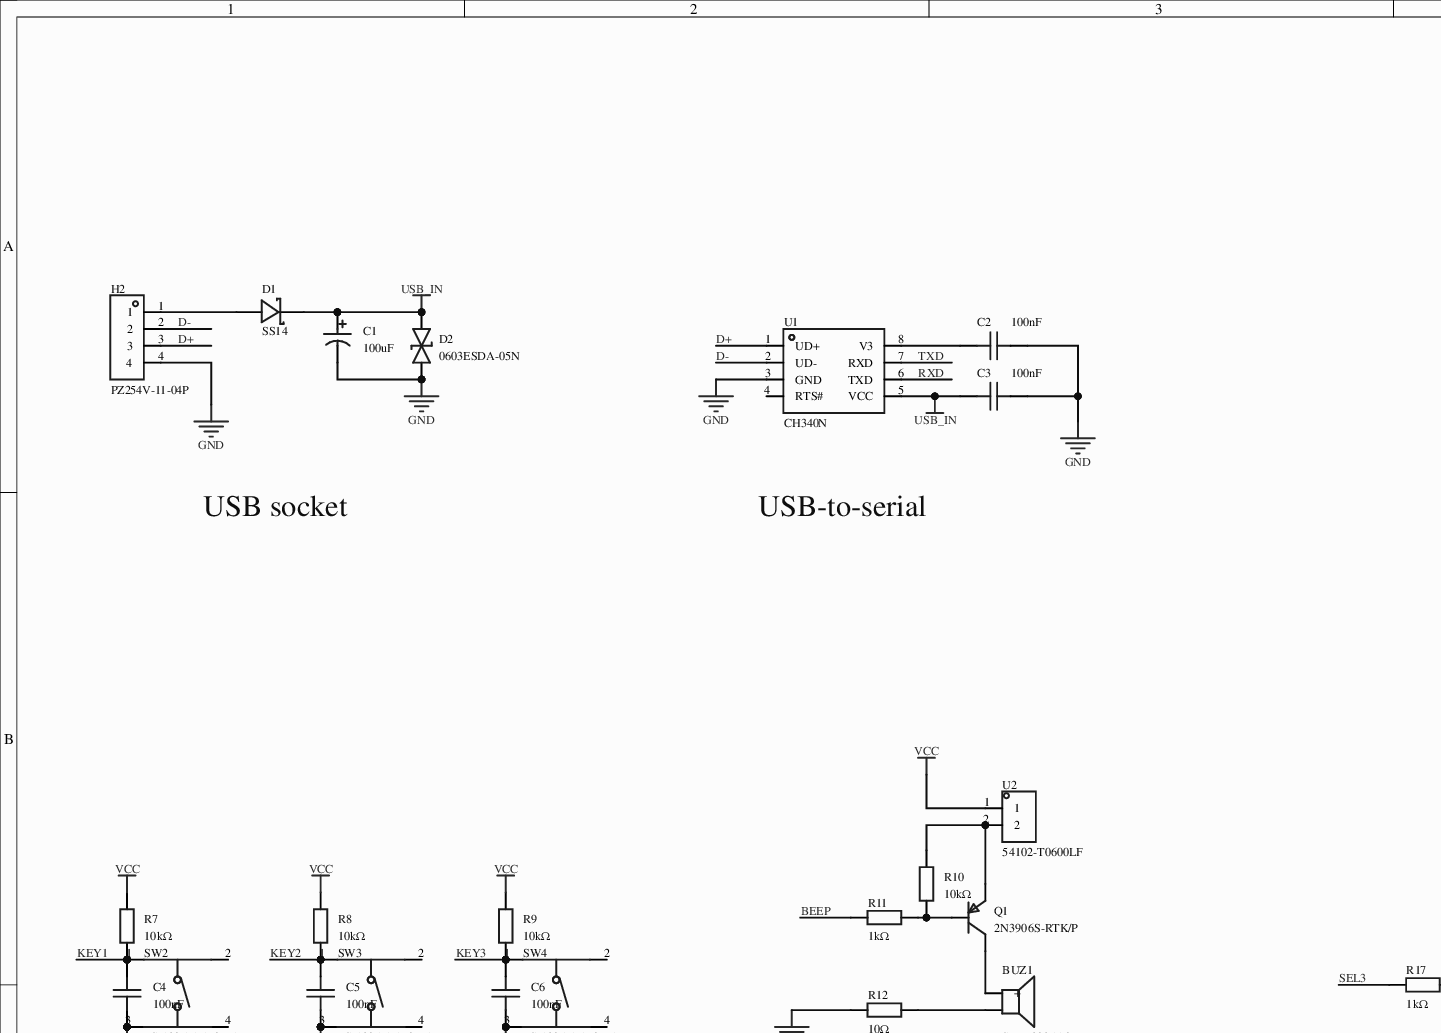
[diagram p0: MISC89012-3.schdoc, top left]
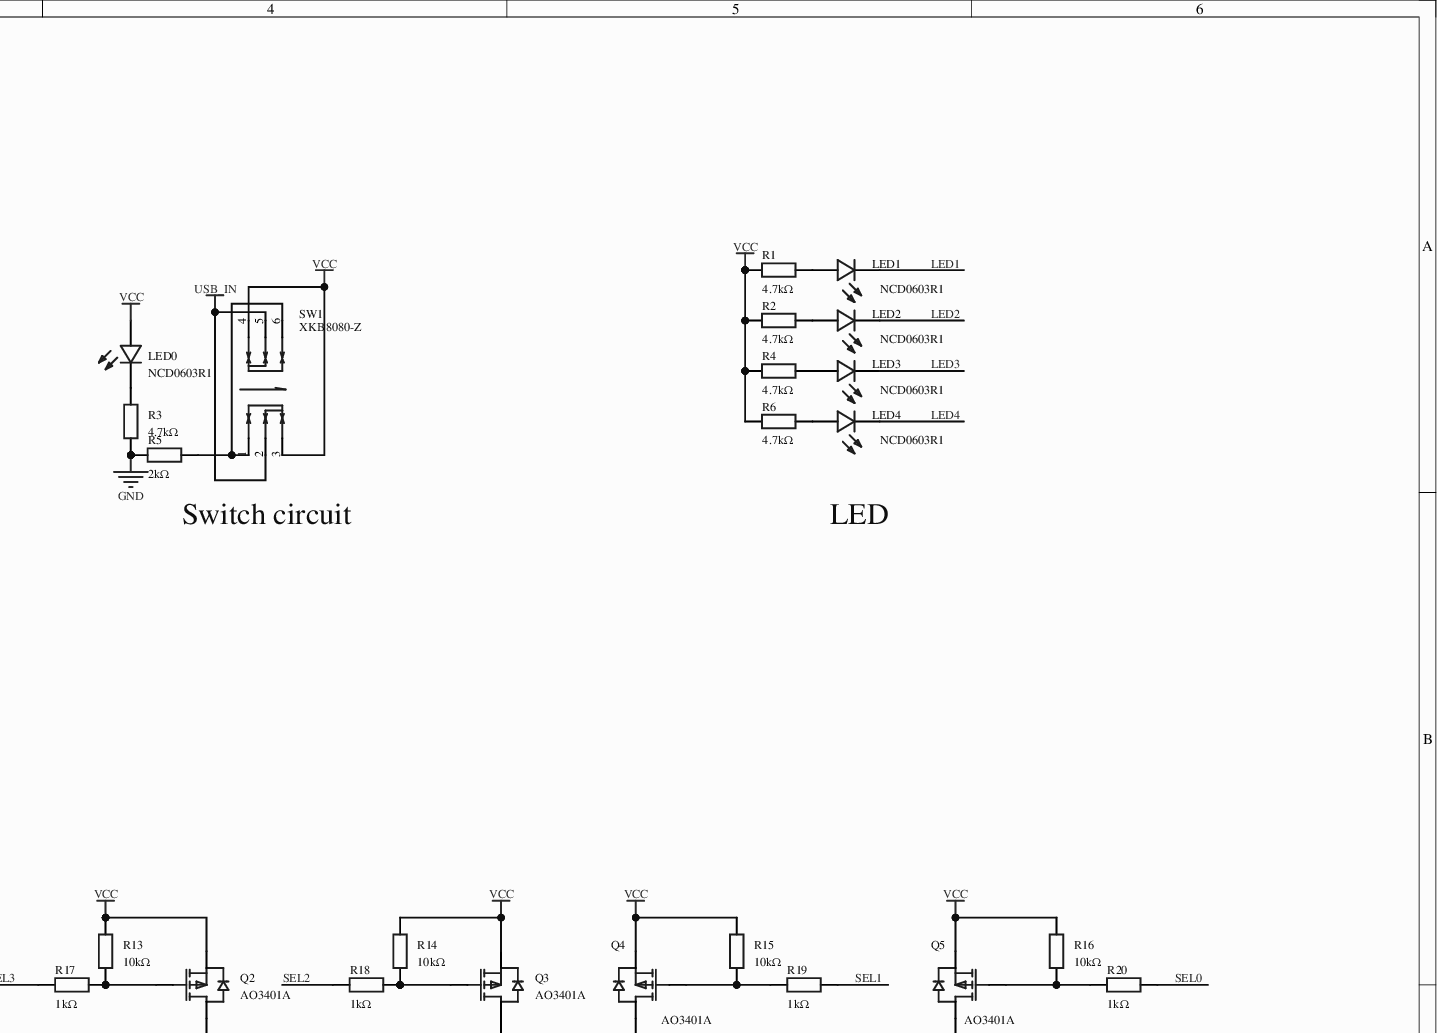
[diagram p1: MISC89012-3.schdoc, top right]
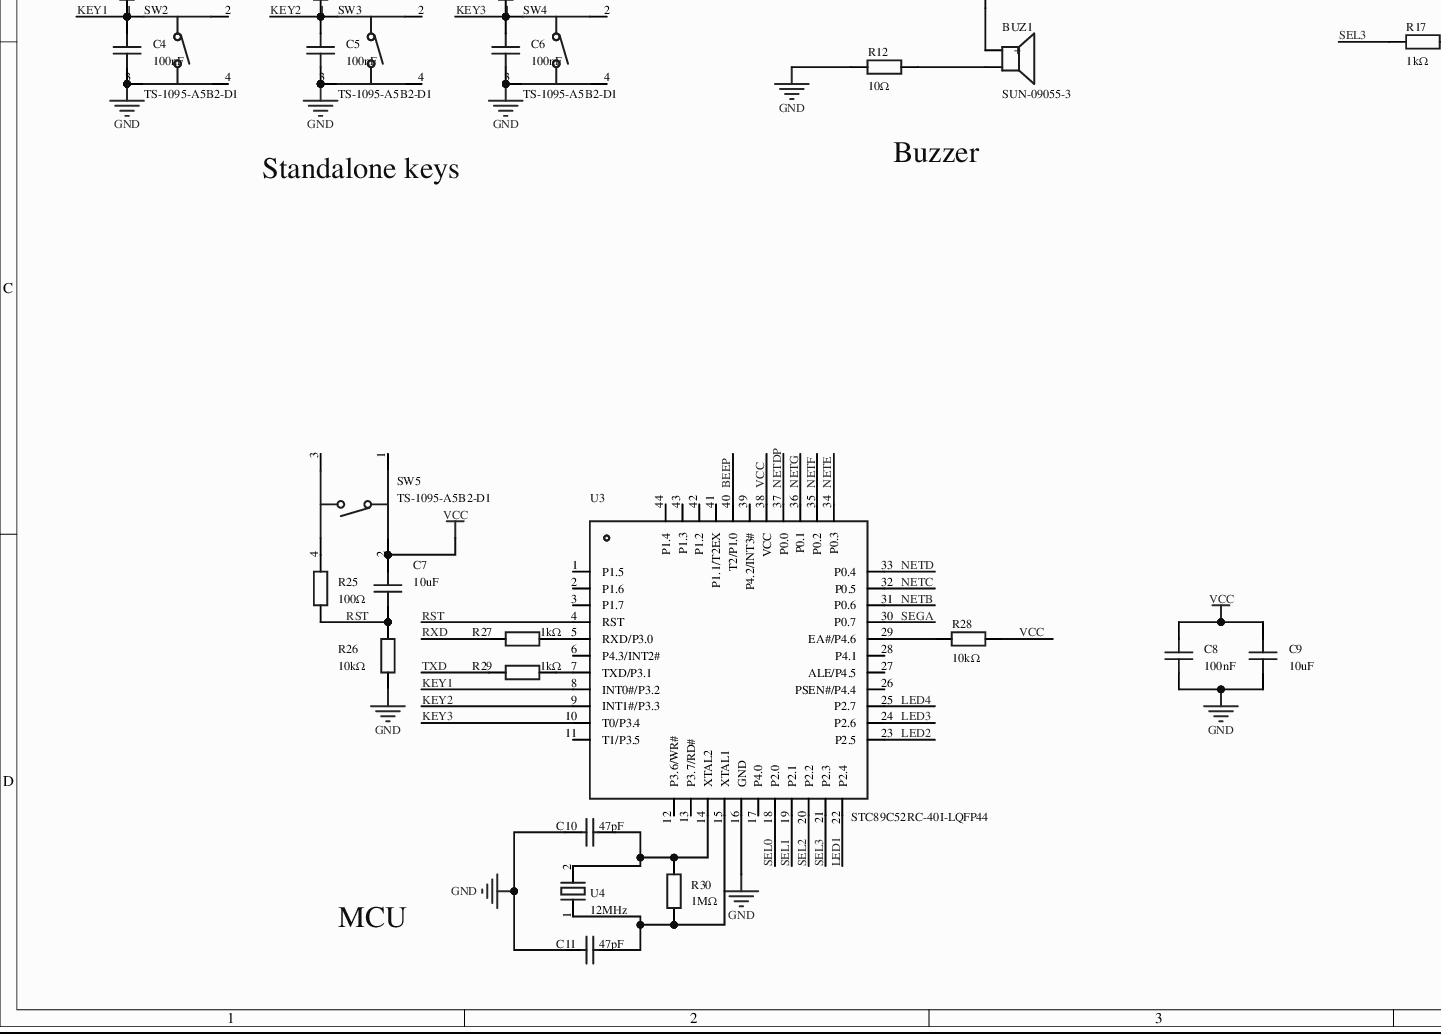
[diagram p2: MISC89012-3.schdoc, bottom left]
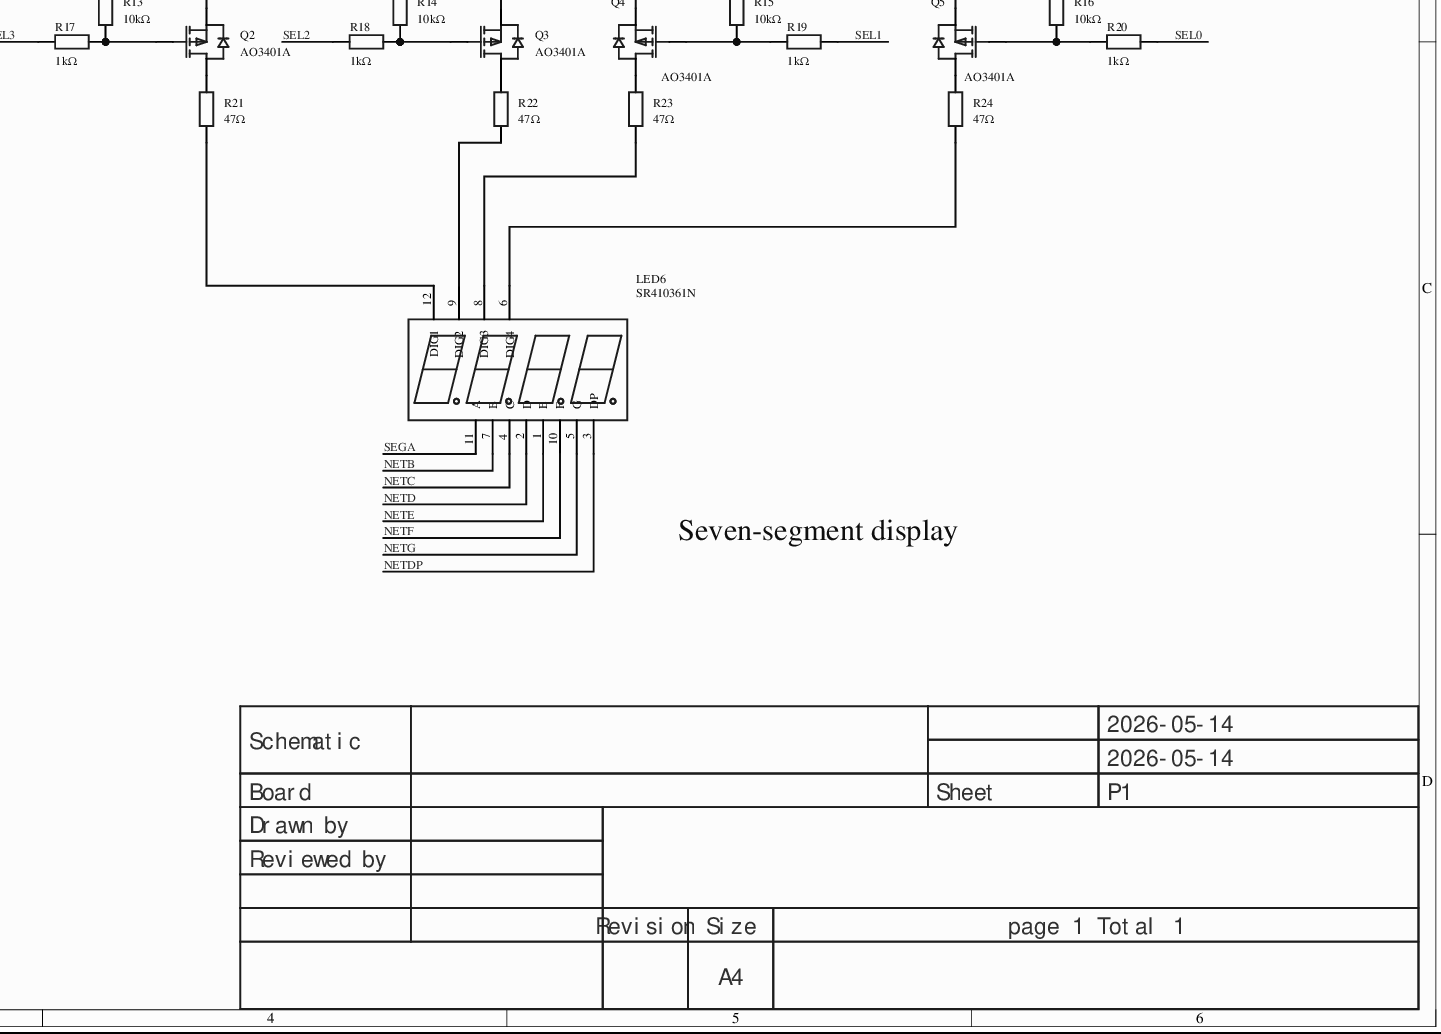
[diagram p3: MISC89012-3.schdoc, bottom right]
# Altium project MISC89012-2.PrjPcb
1 sheet, 65 parts. Net scope: global (net labels, ports and power ports of the same name join across sheets).
Board file: MISC89012.pcbdoc

## Sheet MISC89012-3.schdoc
size 420 x 297 mm; Version: V1.0; @Project Name: MISC89012; @Update Date: 2026-05-14; @Create Date: 2026-05-14; @Board Name: MISC89012; @Create Time: 08:36:15; @Page Count: 1; @Page No: 1; @Schematic Name: MISC89012; @Update Time: 08:36:15; Size: A4

### Parts
BUZ1  SUN-09055-3  [BUZ-TH_BD9.0-P5.00-D0.6-FD]
C1  100uF  [CAP-TH_BD5.0-P2.00-D0.8-FD]
C2  100nF  [C0603]
C3  100nF  [C0603]
C4  100nF  [C0603]
C5  100nF  [C0603]
C6  100nF  [C0603]
C7  10uF  [C0603]
C8  100nF  [C0603]
C9  10uF  [C0603]
C10  47pF  [C0603]
C11  47pF  [C0603]
D1  SS14  [SMA_L4.2-W2.6-LS5.0-RD_1]
D2  0603ESDA-05N  [D0603-BI]
H2  PZ254V-11-04P  [HDR-TH_4P-P2.54-V-M]
LED0  NCD0603R1  [LED0603-RD_RED]
LED1  NCD0603R1  [LED0603-RD_RED]
LED2  NCD0603R1  [LED0603-RD_RED]
LED3  NCD0603R1  [LED0603-RD_RED]
LED4  NCD0603R1  [LED0603-RD_RED]
LED6  SR410361N  [LED-SEG-TH_12P-L30.0-W14.0-P2.54-S10.26-BL]
Q1  2N3906S-RTK/P  [SOT-23-3_L2.9-W1.6-P1.90-LS2.8-TR-CW]
Q2  AO3401A  [SOT-23_L2.9-W1.3-P1.90-LS2.4-BR]
Q3  AO3401A  [SOT-23_L2.9-W1.3-P1.90-LS2.4-BR]
Q4  AO3401A  [SOT-23_L2.9-W1.3-P1.90-LS2.4-BR]
Q5  AO3401A  [SOT-23_L2.9-W1.3-P1.90-LS2.4-BR]
R1  4.7kΩ  [R0603]
R2  4.7kΩ  [R0603]
R3  4.7kΩ  [R0603]
R4  4.7kΩ  [R0603]
R5  2kΩ  [R0603]
R6  4.7kΩ  [R0603]
R7  10kΩ  [R0603]
R8  10kΩ  [R0603]
R9  10kΩ  [R0603]
R10  10kΩ  [R0603]
R11  1kΩ  [R0603]
R12  10Ω  [R0603]
R13  10kΩ  [R0603]
R14  10kΩ  [R0603]
R15  10kΩ  [R0603]
R16  10kΩ  [R0603]
R17  1kΩ  [R0603]
R18  1kΩ  [R0603]
R19  1kΩ  [R0603]
R20  1kΩ  [R0603]
R21  47Ω  [R0603]
R22  47Ω  [R0603]
R23  47Ω  [R0603]
R24  47Ω  [R0603]
R25  100Ω  [R0603]
R26  10kΩ  [R0603]
R27  1kΩ  [R0603]
R28  10kΩ  [R0603]
R29  1kΩ  [R0603]
R30  1MΩ  [R0603]
SW1  XKB8080-Z  [SW-TH_6P-L8.0-W8.0-P2.50]
SW2  TS-1095-A5B2-D1  [SW-TH_4P-L6.0-W6.0-P4.50-LS6.5]
SW3  TS-1095-A5B2-D1  [SW-TH_4P-L6.0-W6.0-P4.50-LS6.5]
SW4  TS-1095-A5B2-D1  [SW-TH_4P-L6.0-W6.0-P4.50-LS6.5]
SW5  TS-1095-A5B2-D1  [SW-TH_4P-L6.0-W6.0-P4.50-LS6.5]
U1  CH340N  [SOP-8_L5.0-W4.0-P1.27-LS6.0-BL]
U2  54102-T0600LF  [HDR-TH_2P-P2.54-V-M-R2-C1-S2.54]
U3  STC89C52RC-40I-LQFP44  [LQFP-44_L10.0-W10.0-P0.80-LS12.0-BL]
U4  12MHz  [HC-49S_L11.4-W4.7-P4.88-D0.4]

### Nets
GND: C1.2 C2.2 C3.2 C4.1 C5.1 C6.1 C8.1 C9.1 C10.1 C11.1 D2.1 H2.4 R3.1 R5.1 R12.1 R26.1 SW2.3 SW3.3 SW4.3 U1.3(GND) U3.16(GND)
USB_IN: C1.1 C3.1 D1.1(K) D2.2 SW1.2 SW1.5 U1.5(VCC)
VCC: C7.2 C8.2 C9.2 LED0.2(A) Q2.2(S) Q3.2(S) Q4.2(S) Q5.2(S) R1.1 R2.1 R4.1 R6.1 R7.2 R8.2 R9.2 R13.2 R14.2 R15.2 R16.2 R28.2 SW1.3 SW1.4 SW5.2 U2.1 U3.38(VCC)
BEEP: R11.1 U3.40(T2/P1.0)
D+: H2.3 U1.1(UD+)
D-: H2.2 U1.2(UD-)
KEY1: C4.2 R7.1 SW2.1 U3.8(INT0#/P3.2)
KEY2: C5.2 R8.1 SW3.1 U3.9(INT1#/P3.3)
KEY3: C6.2 R9.1 SW4.1 U3.10(T0/P3.4)
LED1: LED1.1(K) U3.22(P2.4)
LED2: LED2.1(K) U3.23(P2.5)
LED3: LED3.1(K) U3.24(P2.6)
LED4: LED4.1(K) U3.25(P2.7)
NETB: LED6.7(B) U3.31(P0.6)
NETC: LED6.4(C) U3.32(P0.5)
NETD: LED6.2(D) U3.33(P0.4)
NETDP: LED6.3(DP) U3.37(P0.0)
NETE: LED6.1(E) U3.34(P0.3)
NETF: LED6.10(F) U3.35(P0.2)
NETG: LED6.5(G) U3.36(P0.1)
RST: C7.1 R25.1 R26.2 U3.4(RST)
RXD: R27.1 U1.6(TXD)
SEGA: LED6.11(A) U3.30(P0.7)
SEL0: R20.2 U3.18(P2.0)
SEL1: R19.2 U3.19(P2.1)
SEL2: R18.1 U3.20(P2.2)
SEL3: R17.1 U3.21(P2.3)
TXD: R29.1 U1.7(RXD)
NetBUZ1_1: BUZ1.1(+) Q1.3(C)
NetBUZ1_2: BUZ1.2 R12.2
NetC2_1: C2.1 U1.8(V3)
NetC10_2: C10.2 R30.2 U3.14(XTAL2) U4.2(GND)
NetC11_2: C11.2 R30.1 U3.15(XTAL1) U4.1
NetD1_2: D1.2(A) H2.1
NetLED0_1: LED0.1(K) R3.2
NetLED1_2: LED1.2(A) R1.2
NetLED2_2: LED2.2(A) R2.2
NetLED3_2: LED3.2(A) R4.2
NetLED4_2: LED4.2(A) R6.2
NetLED6_6: LED6.6(DIG4) R24.1
NetLED6_8: LED6.8(DIG3) R23.1
NetLED6_9: LED6.9(DIG2) R22.1
NetLED6_12: LED6.12(DIG1) R21.1
NetQ1_1: Q1.1(E) R10.2 U2.2
NetQ1_2: Q1.2(B) R10.1 R11.2
NetQ2_1: Q2.1(G) R13.1 R17.2
NetQ2_3: Q2.3(D) R21.2
NetQ3_1: Q3.1(G) R14.1 R18.2
NetQ3_3: Q3.3(D) R22.2
NetQ4_1: Q4.1(G) R15.1 R19.1
NetQ4_3: Q4.3(D) R23.2
NetQ5_1: Q5.1(G) R16.1 R20.1
NetQ5_3: Q5.3(D) R24.2
NetR5_2: R5.2 SW1.1 SW1.6
NetR25_2: R25.2 SW5.4
NetR27_2: R27.2 U3.5(RXD/P3.0)
NetR28_1: R28.1 U3.29(EA#/P4.6)
NetR29_2: R29.2 U3.7(TXD/P3.1)

Not connected (* = marked no-connect by the designer): SW2 2* 4*; SW3 2* 4*; SW4 2* 4*; SW5 1* 3*; U1 4(RTS#)*; U3 1(P1.5)* 2(P1.6)* 3(P1.7)* 6(P4.3/INT2#)* 11(T1/P3.5)* 12(P3.6/WR#)* 13(P3.7/RD#)* 17(P4.0)* 26(PSEN#/P4.4)* 27(ALE/P4.5)* 28(P4.1)* 39(P4.2/INT3#)* 41(P1.1/T2EX)* 42(P1.2)* 43(P1.3)* 44(P1.4)*

### Notes on the sheet
- USB socket
- USB-to-serial
- Switch circuit
- LED
- Standalone keys
- Buzzer
- Seven-segment display
- MCU
- 2026-05-14
- Schematic
- Board
- Sheet
- P1
- Drawn by
- Reviewed by
- Revision
- Size
- A4
- page 1 Total 1

### Library data of the parts
BUZ1 = SUN-09055-3: Frequency 2800+300Hz, 1.5-5V voltage drive; AddInBom: yes; ModelId: 13273335caac486e928bafb4d9fdf12d0819f05c4eef4c71ace90d822a990e87; ModelName: BUZ-TH_D9.0-H5.5-P5.0; ModelTransform: 354.33,354.33,0,90,0,0,-0.005,0,-177.165; Symbol: SUN-09055-3; Device: SUN-09055-3; LCSC Part Name: 有源9*5.5  3V; SupplierPart: C47620; ManufacturerPart: SUN-09055-3; Supplier Footprint: 插件; JLCPCB Part Class: Extended Part; Supplier: LCSC; ConvertToPcb: yes; FootprintName: BUZ-TH_BD9.0-P5.00-D0.6-FD
C1 = KS107M016D07RR0VH2FP0: Capacitance: 100uF; Tolerance: ±20%; Rated voltage: 16V; Ripple current: -; ESR: -;; Manufacturer: Chengx(承兴); Symbol: 100uF 16V 5*7; AddInBom: yes; ModelId: edeeed87cbc746108d01291548c386360819f05c4eef4c71ace90d822a990e87; ModelName: CAP-TH_D5.0×H7.0×P2.0; ModelTransform: 197.091,196.7911,0,0,0,0,0,0,-137.795; Pin Spacing: 2mm; Lifetime: 1000hrs@105℃; Device: KS107M016D07RR0VH2FP0; LCSC Part Name: 100uF ±20% 16V; SupplierPart: C43803; ManufacturerPart: KS107M016D07RR0VH2FP0; Supplier Footprint: 插件,D5xL7mm; JLCPCB Part Class: Extended Part; Datasheet: example.com/datasheet/KS107M016D07RR0VH2FP0/44805.html; Supplier: LCSC; ConvertToPcb: yes; FootprintName: CAP-TH_BD5.0-P2.00-D0.8-FD; Value: 100uF; Voltage Rating: 16V; Ripple Current: -; Equivalent Series Resistance(ESR): -; Diameter: 5mm; Height - Seated (Max): 7mm; Operating Temperature: -40℃~+105℃
C2-C6 C8 = CL10B104KB8NNNC: Capacitance: 100nF; Tolerance: ±10%; Rated voltage: 50V; Temperature coefficient: X7R;; Manufacturer: SAMSUNG(三星); AddInBom: yes; ModelId: ac125912035d415993ca9572d50418b10819f05c4eef4c71ace90d822a990e87; ModelName: C0603_L1.6-W0.8-H0.8; ModelTransform: 62.992,31.496,0,0,0,0,0,0,0; Symbol: CL10B104KB8NNNC; Device: CL10B104KB8NNNC; LCSC Part Name: 100nF ±10% 50V; SupplierPart: C1591; ManufacturerPart: CL10B104KB8NNNC; Supplier Footprint: 0603; JLCPCB Part Class: Extended Part; Datasheet: example.com/datasheet/CL10B104KB8NNNC/1943.html; Supplier: LCSC; ConvertToPcb: yes; FootprintName: C0603; Value: 100nF; Voltage Rating: 50V; Temperature Coefficient: X7R
C7 C9 = CL10A106MA8NRNC: Capacitance: 10uF; Tolerance: ±20%; Rated voltage: 25V; Temperature coefficient: X5R;; Manufacturer: SAMSUNG(三星); AddInBom: yes; ModelId: ac125912035d415993ca9572d50418b10819f05c4eef4c71ace90d822a990e87; ModelName: C0603_L1.6-W0.8-H0.8; ModelTransform: 62.992,31.496,0,0,0,0,0,0,0; Symbol: CL10A106MA8NRNC; Device: CL10A106MA8NRNC; LCSC Part Name: 10uF ±20% 25V; SupplierPart: C96446; ManufacturerPart: CL10A106MA8NRNC; Supplier Footprint: 0603; JLCPCB Part Class: Basic Part; Datasheet: example.com/datasheet/CL10A106MA8NRNC/97651.html; Supplier: LCSC; ConvertToPcb: yes; FootprintName: C0603; Value: 10uF; Voltage Rating: 25V; Temperature Coefficient: X5R
C10 C11 = CL10C470JB8NNNC: Capacitance: 47pF; Tolerance: ±5%; Rated voltage: 50V; Temperature coefficient: C0G;; Manufacturer: SAMSUNG(三星); AddInBom: yes; ModelId: ac125912035d415993ca9572d50418b10819f05c4eef4c71ace90d822a990e87; ModelName: C0603_L1.6-W0.8-H0.8; ModelTransform: 62.992,31.496,0,0,0,0,0,0,0; Symbol: CL10C470JB8NNNC; Device: CL10C470JB8NNNC; LCSC Part Name: 47pF ±5% 50V; SupplierPart: C1671; ManufacturerPart: CL10C470JB8NNNC; Supplier Footprint: 0603; JLCPCB Part Class: Basic Part; Datasheet: example.com/datasheet/CL10C470JB8NNNC/2023.html; Supplier: LCSC; ConvertToPcb: yes; FootprintName: C0603; Value: 47pF; Voltage Rating: 50V; Temperature Coefficient: C0G
D1 = SS14_C2480: Diode configuration: Discrete; Forward voltage (Vf): 550mV@1A; DC reverse voltage (Vr): 40V; Rectifier current: 1A;; Manufacturer: MDD(辰达半导体); AddInBom: yes; ModelId: 2ad98c37c5614ad18681cbd22e4725e10819f05c4eef4c71ace90d822a990e87; ModelTransform: 196.85,101.181,0,0,0,0,0,0,0; Reverse Leakage Current (Ir): 300uA@40V; Operating Junction Temperature Range: -55℃~+150℃; Non-Repetitive Peak Forward Surge Current: 25A; Symbol: SS14; Device: SS14_C2480; LCSC Part Name: 电压:40V 电流:1A; SupplierPart: C2480; ManufacturerPart: SS14; Supplier Footprint: SMA(DO-214AC); JLCPCB Part Class: Basic Part; Datasheet: example.com/datasheet/SS14/2857.html; Supplier: LCSC; ConvertToPcb: yes; FootprintName: SMA_L4.2-W2.6-LS5.0-RD_1; ModelName: SMA_L4.2-W2.6-LS5.0-RD_1; Diode Configuration: Discrete; Voltage - Forward(Vf@If): 550mV@1A; Voltage - DC Reverse(Vr): 40V; Current - Rectified: 1A
D2 = 0603ESDA-05N: Polarity: Bidirectional; Reverse standoff voltage (Vrwm): 5V; Clamping voltage: 100V;; Manufacturer: BORN(伯恩半导体); AddInBom: yes; ModelId: a387ce2936f842ebafc868b09fdf8ecc0819f05c4eef4c71ace90d822a990e87; ModelName: DO0603_L1.6-W0.8-H0.8-LS1.6; ModelTransform: 62.992,31.496,0,0,0,0,0,0,0; Reverse Leakage Current (Ir): 500nA; Number of Channels: Single channel; level of protection: IEC 61000-4-2; Type: ESD; Junction Capacitance: 1.5pF; Symbol: 0603ESDA-05N; Device: 0603ESDA-05N; LCSC Part Name: 双向ESD 5V截止; SupplierPart: C316054; ManufacturerPart: 0603ESDA-05N; Supplier Footprint: 0603; JLCPCB Part Class: Extended Part; Datasheet: example.com/datasheet/0603ESDA-05N/297742.html; Supplier: LCSC; ConvertToPcb: yes; FootprintName: D0603-BI; Reverse Stand-Off Voltage (Vrwm): 5V; Clamping Voltage: 100V
H2 = PZ254V-11-04P: Pin structure: 1x4P; Pitch: 2.54mm; Row pitch: -; Round/square pin: Square pin; Mounting type: Through-hole; Number of rows: Single row; Total pins: 4P; Rated current: 3A; Rated voltage: 250V; Mating pin length: 6mm; Housing height: 2.5mm; Termination pin length: 3mm; Contact material: -; Operating temperature: -40℃~+105℃; Color: Black;; Manufacturer: XFCN(兴飞); Symbol: PZ254V-11-04P_C2691448; AddInBom: yes; ModelId: 112f4d05e8d64e99ab9a333894bea4f90819f05c4eef4c71ace90d822a990e87; ModelName: HDR-TH_4P-P2.54-M-LI-1X4P; ModelTransform: 399.999,104.7242,0,0,0,0,0,0,-118.11; Device: PZ254V-11-04P; LCSC Part Name: 1x4P 间距:2.54mm 方针 直插; SupplierPart: C2691448; ManufacturerPart: PZ254V-11-04P; Supplier Footprint: 插件,P=2.54mm; JLCPCB Part Class: Extended Part; Datasheet: example.com/datasheet/PZ254V-11-04P/2801085.html; Supplier: LCSC; ConvertToPcb: yes; FootprintName: HDR-TH_4P-P2.54-V-M; Pin Structure: 1x4P; Row Spacing: -; Circluar Pins/Square Pins: Square pin; Mounting Type: Through-hole; Number of Rows: Single row; Number of Pins: 4P; Current Rating: 3A; Voltage Rating (Max): 250V; Length of Mating Pin: 6mm; Insulation Height: 2.5mm; Length of End Connection Pin: 3mm; Contact Material: -; Operating Temperature: -40℃~+105℃; Color: Black
LED0-LED4 = NCD0603R1_C84263: LED package type: -; Emission color: Red; Forward voltage (Vf): 1.6V~2.6V; Power: 65mW; Forward current: 25mA; Wavelength: 615nm~630nm; Diode configuration: Discrete diode; Lens color: -; Color temperature: -; Luminous intensity: 220mcd; Viewing angle: 130°; Packaging: -; Operating temperature: -30℃~+85℃;; Manufacturer: 国星光电; Symbol: FC-DA1608HRK-620D; AddInBom: yes; ModelId: 74041d3a270d435c8600a9ab9b7641c00819f05c4eef4c71ace90d822a990e87; ModelTransform: 63.7794,31.496,0,0,0,0,0,-0.002,0; Peak Wavelength: 630nm; Device: NCD0603R1_C84263; LCSC Part Name: 片式发光二极管; SupplierPart: C84263; ManufacturerPart: NCD0603R1; Supplier Footprint: 0603; JLCPCB Part Class: Extended Part; Datasheet: example.com/datasheet/NCD0603R1/85432.html; Supplier: LCSC; ConvertToPcb: yes; FootprintName: LED0603-RD_RED; ModelName: LED0603-RD_RED; Lamp Holder Type: -; Illumination Color: Red; Voltage - Forward(Vf): 1.6V~2.6V; Power(Watts): 65mW; Forward Current: 25mA; Wavelength - Dominant: 615nm~630nm; Diode Configuration: Discrete diode; Lens Color: -; Color Temperature: -; Luminous Intensity: 220mcd; Viewing Angle: 130°; Mounting Style: -; Operating Temperature: -30℃~+85℃
LED6 = SR410361N: Digits: 4-digit; Character size (inch): 0.36; LED polarity: Common anode; Emission color: Red; Power dissipation (Pd): 50mW;; Manufacturer: ARKLED(方舟); Symbol: SR410361N_1; AddInBom: yes; ModelId: b3ca015d840f48199c94aa3009a97aa80819f05c4eef4c71ace90d822a990e87; ModelName: LED-SEG-TH_12P-L30.0-W14.0-H7.2-P2.54-S10.26-BL; ModelTransform: 1181.1,551.18,0,0,0,0,0,0,-196.85; Digit/Alpha Size(inch): 0.36; Display Type: 7-segment; Light Intensity: 25mcd; Forward Voltage Drop: 2V; Device: SR410361N; LCSC Part Name: 4位0.36英寸红色数码管 共阳极; SupplierPart: C132660; ManufacturerPart: SR410361N; Supplier Footprint: 插件; JLCPCB Part Class: Extended Part; Datasheet: example.com/datasheet/SR410361N/143960.html; Supplier: LCSC; ConvertToPcb: yes; FootprintName: LED-SEG-TH_12P-L30.0-W14.0-P2.54-S10.26-BL; Number of Characters: 4-digit; LED Polarity: Common anode; Illumination Color: Red; Pd - Power Dissipation: 50mW; Operating Temperature: -20℃~+80℃; Length: 30mm; Width: 14mm; Height: 7.2mm
Q1 = 2N3906S-RTK/P_C147294: Transistor type: PNP; Collector current (Ic): 200mA; Collector-emitter breakdown voltage (Vceo): 40V; Power dissipation (Pd): 350mW; DC current gain (hFE): 100@10mA,1V;; Manufacturer: KEC; Symbol: 2N3906S-RTK/PS; AddInBom: yes; ModelId: 057a289c59fb43c9b236341d87f3a1af0819f05c4eef4c71ace90d822a990e87; ModelTransform: 114.173,110.236,0,90,0,0,0,0,0; Transition frequency(fT): 250MHz; Current - Collector Cutoff: 50nA; Vce Saturation(VCE(sat)): 400mV@50mA,5mA; Emitter-Base Voltage(Vebo): 5V; Device: 2N3906S-RTK/P_C147294; LCSC Part Name: PNP 电流:200mA 电压:40V; SupplierPart: C147294; ManufacturerPart: 2N3906S-RTK/P; Supplier Footprint: SOT-23; JLCPCB Part Class: Extended Part; Datasheet: example.com/datasheet/2N3906S-RTK%252FP/158626.html; Supplier: LCSC; ConvertToPcb: yes; FootprintName: SOT-23-3_L2.9-W1.6-P1.90-LS2.8-TR-CW; ModelName: SOT-23-3_L2.9-W1.6-P1.90-LS2.8-TR-CW; type: PNP; Current - Collector(Ic): 200mA; Collector - Emitter Voltage VCEO: 40V; Pd - Power Dissipation: 350mW; DC Current Gain: 100@10mA,1V; Operating Temperature: -
Q2-Q5 = AO3401A_C15127: 数量:1个P沟道;漏源电压(Vdss):30V;连续漏极电流(Id):4A;导通电阻(RDS(on)):47mΩ@10V；85mΩ@2.5V；60mΩ@4.5V;耗散功率(Pd):-;阈值电压(Vgs(th)):900mV;; Manufacturer: AOS; AddInBom: yes; ModelId: c62791f0466c4ae2a892c056b845b0ca0819f05c4eef4c71ace90d822a990e87; ModelName: SOT-23-3P_L2.9-W1.3-H1.0-LS2.4-P0.95; ModelTransform: 98.64468,114.173,0,180,0,0,0.001,-0.002,0; Number: 1个P沟道; Drain to Source Voltage: 30V; Current - Continuous Drain(Id): 4A; RDS(on): 47mΩ@10V; 85mΩ@2.5V; 60mΩ@4.5V; Gate Threshold Voltage (Vgs(th)): 900mV; Gate Charge(Qg): 14nC@10V; Input Capacitance(Ciss): 645pF; Reverse Transfer Capacitance (Crss@Vds): 55pF; Output Capacitance(Coss): 80pF; Symbol: AO3401A; Device: AO3401A_C15127; LCSC Part Name: 1个P沟道 耐压:30V 电流:4A; SupplierPart: C15127; ManufacturerPart: AO3401A; Supplier Footprint: SOT-23; JLCPCB Part Class: Basic Part; Datasheet: example.com/datasheet/AO3401A/15801.html; Supplier: LCSC; ConvertToPcb: yes; FootprintName: SOT-23_L2.9-W1.3-P1.90-LS2.4-BR; Pd - Power Dissipation: -; Operating Temperature: -; Type: -
R1-R4 R6 = RC0603FR-074K7L: Resistor type: Thick-film resistor; Resistance: 4.7kΩ; Tolerance: ±1%; Power: 100mW; Operating voltage: 75V; Temperature coefficient: ±100ppm/℃;; Manufacturer: YAGEO(国巨); AddInBom: yes; ModelId: fc143cca1e79419f9cd78b61e9279f080819f05c4eef4c71ace90d822a990e87; ModelTransform: 31.8897,63.7794,0,90,0,0,0,0,0; Symbol: RC0603FR-074K7L; Device: RC0603FR-074K7L; LCSC Part Name: 厚膜电阻 4.7kΩ ±1% 100mW; SupplierPart: C99782; ManufacturerPart: RC0603FR-074K7L; Supplier Footprint: 0603; JLCPCB Part Class: Extended Part; Datasheet: example.com/datasheet/RC0603FR-074K7L/100996.html; Supplier: LCSC; ConvertToPcb: yes; FootprintName: R0603; ModelName: R0603; Type: Thick-film resistor; Value: 4.7kΩ; Power(Watts): 100mW; Voltage-Supply(Max): 75V; Temperature Coefficient: ±100ppm/℃; Operating Temperature: -55℃~+155℃
R5 = 0603WAF2001T5E: Resistor type: Thick-film resistor; Resistance: 2kΩ; Tolerance: ±1%; Power: 100mW; Operating voltage: 75V; Temperature coefficient: ±100ppm/℃;; Manufacturer: UNI-ROYAL(厚声); AddInBom: yes; ModelId: fc143cca1e79419f9cd78b61e9279f080819f05c4eef4c71ace90d822a990e87; ModelTransform: 31.8897,63.7794,0,90,0,0,0,0,0; Symbol: 0603WAF2001T5E; Device: 0603WAF2001T5E; LCSC Part Name: 2kΩ ±1% 100mW 厚膜电阻; SupplierPart: C22975; ManufacturerPart: 0603WAF2001T5E; Supplier Footprint: 0603; JLCPCB Part Class: Basic Part; Datasheet: example.com/datasheet/0603WAF2001T5E/23702.html; Supplier: LCSC; ConvertToPcb: yes; FootprintName: R0603; ModelName: R0603; Type: Thick-film resistor; Value: 2kΩ; Power(Watts): 100mW; Voltage-Supply(Max): 75V; Temperature Coefficient: ±100ppm/℃; Operating Temperature: -55℃~+155℃
R7-R10 R13-R16 R26 R28 = 0603WAF1002T5E: Resistor type: Thick-film resistor; Resistance: 10kΩ; Tolerance: ±1%; Power: 100mW; Operating voltage: 75V; Temperature coefficient: ±100ppm/℃;; Manufacturer: UNI-ROYAL(厚声); AddInBom: yes; ModelId: fc143cca1e79419f9cd78b61e9279f080819f05c4eef4c71ace90d822a990e87; ModelTransform: 31.8897,63.7794,0,90,0,0,0,0,0; Symbol: 0603WAF1002T5E; Device: 0603WAF1002T5E; LCSC Part Name: 厚膜电阻 10kΩ ±1% 100mW; SupplierPart: C25804; ManufacturerPart: 0603WAF1002T5E; Supplier Footprint: 0603; JLCPCB Part Class: Basic Part; Datasheet: example.com/datasheet/0603WAF1002T5E/26547.html; Supplier: LCSC; ConvertToPcb: yes; FootprintName: R0603; ModelName: R0603; Type: Thick-film resistor; Value: 10kΩ; Power(Watts): 100mW; Voltage-Supply(Max): 75V; Temperature Coefficient: ±100ppm/℃; Operating Temperature: -55℃~+155℃
R11 R17-R20 R27 R29 = RC0603FR-071KL: Resistor type: Thick-film resistor; Resistance: 1kΩ; Tolerance: ±1%; Power: 100mW; Operating voltage: 75V; Temperature coefficient: ±100ppm/℃;; Manufacturer: YAGEO(国巨); AddInBom: yes; ModelId: fc143cca1e79419f9cd78b61e9279f080819f05c4eef4c71ace90d822a990e87; ModelTransform: 31.8897,63.7794,0,90,0,0,0,0,0; Symbol: RC0603FR-071KL; Device: RC0603FR-071KL; LCSC Part Name: 厚膜电阻 1kΩ ±1% 100mW; SupplierPart: C22548; ManufacturerPart: RC0603FR-071KL; Supplier Footprint: 0603; JLCPCB Part Class: Extended Part; Datasheet: example.com/datasheet/RC0603FR-071KL/23274.html; Supplier: LCSC; ConvertToPcb: yes; FootprintName: R0603; ModelName: R0603; Type: Thick-film resistor; Value: 1kΩ; Power(Watts): 100mW; Voltage-Supply(Max): 75V; Temperature Coefficient: ±100ppm/℃; Operating Temperature: -55℃~+155℃
R12 = 0603WAF100JT5E: Resistor type: Thick-film resistor; Resistance: 10Ω; Tolerance: ±1%; Power: 100mW; Operating voltage: 75V; Temperature coefficient: ±400ppm/℃;; Manufacturer: UNI-ROYAL(厚声); AddInBom: yes; ModelId: fc143cca1e79419f9cd78b61e9279f080819f05c4eef4c71ace90d822a990e87; ModelTransform: 31.8897,63.7794,0,90,0,0,0,0,0; Symbol: 0603WAF100JT5E; Device: 0603WAF100JT5E; LCSC Part Name: 10Ω ±1% 100mW 厚膜电阻; SupplierPart: C22859; ManufacturerPart: 0603WAF100JT5E; Supplier Footprint: 0603; JLCPCB Part Class: Basic Part; Datasheet: example.com/datasheet/0603WAF100JT5E/23586.html; Supplier: LCSC; ConvertToPcb: yes; FootprintName: R0603; ModelName: R0603; Type: Thick-film resistor; Value: 10Ω; Power(Watts): 100mW; Voltage-Supply(Max): 75V; Temperature Coefficient: ±400ppm/℃; Operating Temperature: -55℃~+155℃
R21-R24 = 0603WAF470JT5E: Resistor type: Thick-film resistor; Resistance: 47Ω; Tolerance: ±1%; Power: 100mW; Operating voltage: 75V; Temperature coefficient: ±100ppm/℃;; Manufacturer: UNI-ROYAL(厚声); AddInBom: yes; ModelId: fc143cca1e79419f9cd78b61e9279f080819f05c4eef4c71ace90d822a990e87; ModelTransform: 31.8897,63.7794,0,90,0,0,0,0,0; Symbol: 0603WAF470JT5E; Device: 0603WAF470JT5E; LCSC Part Name: 47Ω ±1% 100mW 厚膜电阻; SupplierPart: C23182; ManufacturerPart: 0603WAF470JT5E; Supplier Footprint: 0603; JLCPCB Part Class: Basic Part; Datasheet: example.com/datasheet/0603WAF470JT5E/23909.html; Supplier: LCSC; ConvertToPcb: yes; FootprintName: R0603; ModelName: R0603; Type: Thick-film resistor; Value: 47Ω; Power(Watts): 100mW; Voltage-Supply(Max): 75V; Temperature Coefficient: ±100ppm/℃; Operating Temperature: -55℃~+155℃
R25 = RC0603FR-07100RL: Resistor type: Thick-film resistor; Resistance: 100Ω; Tolerance: ±1%; Power: 100mW; Max operating voltage: 75V; Temperature coefficient: ±100ppm/℃;; Manufacturer: YAGEO(国巨); AddInBom: yes; ModelId: fc143cca1e79419f9cd78b61e9279f080819f05c4eef4c71ace90d822a990e87; ModelTransform: 31.8897,63.7794,0,90,0,0,0,0,0; Symbol: RC0603FR-07100RL; Device: RC0603FR-07100RL; LCSC Part Name: 厚膜电阻 100Ω ±1% 100mW; SupplierPart: C105588; ManufacturerPart: RC0603FR-07100RL; Supplier Footprint: 0603; JLCPCB Part Class: Extended Part; Datasheet: example.com/upload/public/pdf/source/20180316/70C0E2BDAE7FCC62C531A5A58D202EE1.pdf; Supplier: LCSC; ConvertToPcb: yes; FootprintName: R0603; ModelName: R0603; Type: Thick-film resistor; Value: 100Ω; Power(Watts): 100mW; Overload Voltage (Max): 75V; Temperature Coefficient: ±100ppm/℃; Operating Temperature Range: -55℃~+155℃
R30 = 0603WAF1004T5E: Resistor type: Thick-film resistor; Resistance: 1MΩ; Tolerance: ±1%; Power: 100mW; Max operating voltage: 75V; Temperature coefficient: ±100ppm/℃;; Manufacturer: UNI-ROYAL(厚声); AddInBom: yes; ModelId: fc143cca1e79419f9cd78b61e9279f080819f05c4eef4c71ace90d822a990e87; ModelTransform: 31.8897,63.7794,0,90,0,0,0,0,0; Symbol: 0603WAF1004T5E; Device: 0603WAF1004T5E; LCSC Part Name: 1MΩ ±1% 100mW 厚膜电阻; SupplierPart: C22935; ManufacturerPart: 0603WAF1004T5E; Supplier Footprint: 0603; JLCPCB Part Class: Basic Part; Datasheet: example.com/upload/public/pdf/source/20200306/C422600_1E6D84923E4A46A82E41ADD87F860B5C.pdf; Supplier: LCSC; ConvertToPcb: yes; FootprintName: R0603; ModelName: R0603; Type: Thick-film resistor; Value: 1MΩ; Power(Watts): 100mW; Overload Voltage (Max): 75V; Temperature Coefficient: ±100ppm/℃; Operating Temperature Range: -55℃~+155℃
SW1 = XKB8080-Z: Latching/non-latching: Latching; Mounting type: Through-hole; Contact current: 100mA; Rated voltage: 30V; With lamp: Without; Actuating force: 1.6N; Operating life: 10万 cycles;; Manufacturer: XKB Connection(中国星坤); AddInBom: yes; ModelId: 2ca63b555ed647238a13c4f5c29203120819f05c4eef4c71ace90d822a990e87; ModelName: SW-TH_L8.0-W8.0-H13.7-P2.5; ModelTransform: 314.96,314.96,0,90,0,0,0,0,-125.984; Actuator Style: Rectangular button; Actuator/Cap Color: Blue; Symbol: XKB8080-Z; Device: XKB8080-Z; LCSC Part Name: 8*8 蓝白黑 自锁开关; SupplierPart: C318860; ManufacturerPart: XKB8080-Z; Supplier Footprint: 插件; JLCPCB Part Class: Extended Part; Datasheet: example.com/datasheet/XKB8080-Z/299952.html; Supplier: LCSC; ConvertToPcb: yes; FootprintName: SW-TH_6P-L8.0-W8.0-P2.50; Self Lock / No Lock: Latching; IP Rating: -; Mounting Type: Through-hole; Contact Current: 100mA; Voltage Rating: 30V; With Lamp: Without; Termination Style: PC pin; Operating Force: 1.6N; Operating Temperature: -15℃~+55℃; Life: 10万 cycles
SW2-SW5 = TS-1095-A5B2-D1: Circuit configuration: SPST; Button shape: Round button; Actuating force: 180gf; Mounting type: Through-hole; Switch length: 6mm; Switch width: 6mm; Switch height: 6mm; With bracket: Without; Mechanical life: -;; Manufacturer: Yuandi(元迪); AddInBom: yes; ModelId: 20eee248bc684ccd8cbdbb1d0d91ec6f0819f05c4eef4c71ace90d822a990e87; ModelName: SW-TH_4P-L6.0-W6.0-H5.0-LS6.5-P4.50; ModelTransform: 236.22,323.03,0,90,0,0,0,0,-137.795; Actuator/Cap Color: Black; Pin Style: PC pin; Symbol: TS-1095-A5B2-D1; Device: TS-1095-A5B2-D1; LCSC Part Name: 6*6*6mm 直插 轻触开关; SupplierPart: C782808; ManufacturerPart: TS-1095-A5B2-D1; Supplier Footprint: 插件; JLCPCB Part Class: Extended Part; Datasheet: example.com/upload/public/pdf/source/20200908/C782804_D14F61DCCBE05C7EE913124CF28857B3.pdf; Supplier: LCSC; ConvertToPcb: yes; FootprintName: SW-TH_4P-L6.0-W6.0-P4.50-LS6.5; Circuit: SPST; Actuator Style: Round button; Operating Force: 180gf; Mounting Style: Through-hole; Switch Length: 6mm; Switch Width: 6mm; Switch Height: 6mm; Strike Gundam: Without; Mechanical Life: -
U1 = CH340N_C506813: Function: USB-to-serial; Interface protocol: USB 2.0; Channels: -; Data rate: 2Mbps;; Manufacturer: WCH(南京沁恒); AddInBom: yes; ModelId: a3315c1c78f949e6bb82c6eaca1c53c70819f05c4eef4c71ace90d822a990e87; ModelName: SOP-8_L5.0-W4.0-H1.8-LS6.2-P1.27; ModelTransform: 244.094,196.85,0,90,0,0,0,0,0; Protocol: USB 2.0; Supply Voltage: 3.3V; 5V; Symbol: CH340N; Device: CH340N_C506813; LCSC Part Name: USB转串口芯片CH340; SupplierPart: C506813; ManufacturerPart: CH340N; Supplier Footprint: SOP-8; JLCPCB Part Class: Extended Part; Datasheet: example.com/upload/public/pdf/source/20200819/C84681_ADBED554CE321879DBD6B1D06488689C.pdf; Supplier: LCSC; ConvertToPcb: yes; FootprintName: SOP-8_L5.0-W4.0-P1.27-LS6.0-BL; Applications Function: USB-to-serial; Number of Channels: -; Data Rate: 2Mbps; Operating Temperature: -20℃~+70℃
U2 = 54102-T0600LF: Pin structure: -; Pitch: 2.54mm; Row pitch: 2.54mm; Round/square pin: Square pin; Mounting type: Through-hole; Number of rows: Double row; Rated current: 3A; Rated voltage: -; Mating pin length: 5.84mm; Housing height: 2.54mm; Termination pin length: 2.79mm; Contact material: Phosphor bronze; Contact plating: Tin; Operating temperature: -65℃~+125℃; Color: Black;; Manufacturer: Amphenol; AddInBom: yes; ModelId: 5349b451ee304bceb48a29b5d747cdd10819f05c4eef4c71ace90d822a990e87; ModelName: HDR-TH_2P-P2.54-M-LI-2X1P; ModelTransform: 100,190.1571,0,0,0,0,0,0,-118.11; Symbol: 54102-T0600LF; Device: 54102-T0600LF; LCSC Part Name: 间距:2.54mm 方针 直插; SupplierPart: C213465; ManufacturerPart: 54102-T0600LF; Supplier Footprint: 插件,P=2.54mm; JLCPCB Part Class: Extended Part; Datasheet: example.com/datasheet/54102-T0600LF/214372.html; Supplier: LCSC; ConvertToPcb: yes; FootprintName: HDR-TH_2P-P2.54-V-M-R2-C1-S2.54; Pin Structure: -; Row Spacing: 2.54mm; Circluar Pins/Square Pins: Square pin; Mounting Type: Through-hole; Number of Rows: Double row; Current Rating: 3A; Voltage Rating (Max): -; Length of Mating Pin: 5.84mm; Insulation Height: 2.54mm; Length of End Connection Pin: 2.79mm; Contact Material: Phosphor bronze; Contact Plating: Tin; Operating Temperature: -65℃~+125℃; Color: Black
U3 = STC89C52RC-40I-LQFP44: CPU core: 51 family;; Manufacturer: STC; Symbol: STC89C52RC-40I_C8707; AddInBom: yes; ModelId: cfc67ede9fd147078f17820e55193bca0819f05c4eef4c71ace90d822a990e87; ModelName: LQFP-44_L10.0-W10.0-H1.4-LS12.0-P0.80; ModelTransform: 472.441,472.441,0,0,0,0,0,0,0; Program Storage Size: 8KB; Program Memory Type: FLASH; Number of I/O: 39; Voltage - Supply: 3.3V~5.5V; Device: STC89C52RC-40I-LQFP44; LCSC Part Name: 单片机原理及应用; SupplierPart: C8707; ManufacturerPart: STC89C52RC-40I-LQFP44; Supplier Footprint: LQFP-44(10x10); JLCPCB Part Class: Extended Part; Datasheet: example.com/datasheet/STC89C52RC-40I-LQFP44/9213.html; Supplier: LCSC; ConvertToPcb: yes; FootprintName: LQFP-44_L10.0-W10.0-P0.80-LS12.0-BL; CPU Core: 51 family
U4 = 049ST2-12.000F18DTLJL: Crystal type: Through-hole crystal; Frequency: 12MHz; Frequency tolerance at room temperature: ±20ppm; Load capacitance: 18pF; Frequency stability: ±30ppm;; Manufacturer: HCI(杭晶); AddInBom: yes; ModelId: ed749e7777a548268de10898a0bd374a0819f05c4eef4c71ace90d822a990e87; ModelTransform: 445.84659,183.0705,0,0,0,0,0,0,-137.795; Equivalent Series Resistance(ESR): 50Ω; Symbol: 049ST2-12.000F18DTLJL; Device: 049ST2-12.000F18DTLJL; LCSC Part Name: HC-49S 2P 12MHz 18pF ±20ppm -40~+85℃(±30ppm); SupplierPart: C19674272; ManufacturerPart: 049ST2-12.000F18DTLJL; Supplier Footprint: HC-49S-2P; JLCPCB Part Class: Extended Part; Datasheet: example.com/datasheet/049ST2-12.000F18DTLJL/20981424.html; Supplier: LCSC; ConvertToPcb: yes; FootprintName: HC-49S_L11.4-W4.7-P4.88-D0.4; ModelName: HC-49S_L11.4-W4.7-P4.88-D0.4; Type: Through-hole crystal; Value: 12MHz; Normal temperature Frequency Tolerance: ±20ppm; Load Capacitance: 18pF; Frequency Stability: ±30ppm; Operating Temperature: -40℃~+85℃